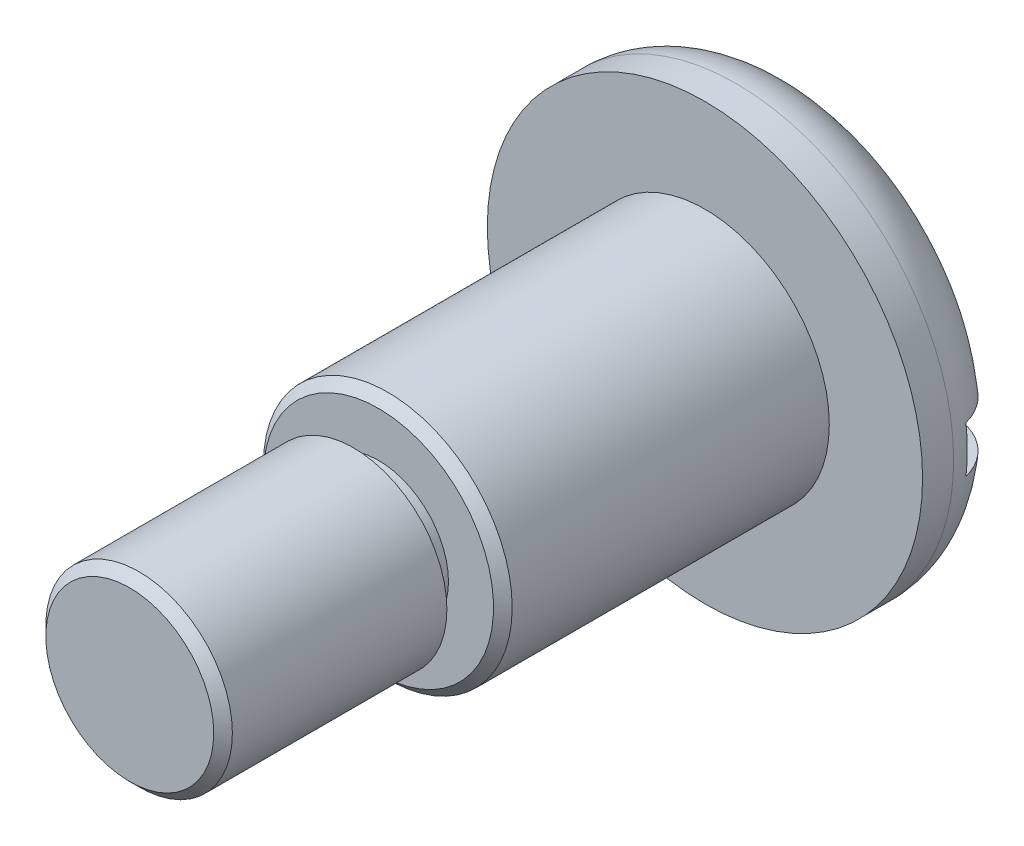
from build123d import *

# Parameters (mm, degrees)
SKETCH_1_R          = 7
EXTRUDE_1_DEPTH     = 3
SKETCH_2_R          = 4
EXTRUDE_2_DEPTH     = 10.5
SKETCH_3_R          = 3
EXTRUDE_3_DEPTH     = 8
SKETCH_4_R          = 3
SKETCH_4_R_2        = 2.25
CUT_EXTRUDE_1_DEPTH = 0.8
FILLET_1_R          = 2
SKETCH_5_W          = 17.035496118
SKETCH_5_H          = 1.5
CUT_EXTRUDE_2_DEPTH = 1.5
CHAMFER_1_SIZE      = 0.3


with BuildPart() as part:
    # 草图1 → 凸台-拉伸1 (new body)
    with BuildSketch(Plane.XY):
        Circle(SKETCH_1_R)
    extrude(amount=EXTRUDE_1_DEPTH)

    # 草图2 → 凸台-拉伸2 (add)
    with BuildSketch(Plane.XY.offset(3)):
        with Locations(Location((0, 0, 0), (0, 0, 180))):
            Circle(SKETCH_2_R)
    extrude(amount=EXTRUDE_2_DEPTH)

    # 草图3 → 凸台-拉伸3 (add)
    with BuildSketch(Plane.XY.offset(13.5)):
        Circle(SKETCH_3_R)
    extrude(amount=EXTRUDE_3_DEPTH)

    # 草图4 → 切除-拉伸1 (cut)
    with BuildSketch(Plane.XY.offset(13.5)):
        Circle(SKETCH_4_R)
        Circle(SKETCH_4_R_2, mode=Mode.SUBTRACT)
    extrude(amount=CUT_EXTRUDE_1_DEPTH, mode=Mode.SUBTRACT)

    # 圆角1
    fillet_1_edges = [part.edges().sort_by_distance(p)[0] for p in [
        (-7, 0, 0),
    ]]
    fillet(fillet_1_edges, radius=FILLET_1_R)

    # 草图5 → 切除-拉伸2 (cut)
    with BuildSketch(Plane(origin=(0, 0, 0), x_dir=(-1, 0, 0), z_dir=(0, 0, -1))):
        Rectangle(SKETCH_5_W, SKETCH_5_H)
    extrude(amount=-CUT_EXTRUDE_2_DEPTH, mode=Mode.SUBTRACT)

    # 倒角1
    chamfer_1_edges = [part.edges().sort_by_distance(p)[0] for p in [
        (-3, 0, 21.5),
        (4, 0, 13.5),
    ]]
    chamfer(chamfer_1_edges, length=CHAMFER_1_SIZE)


solid = part.part
